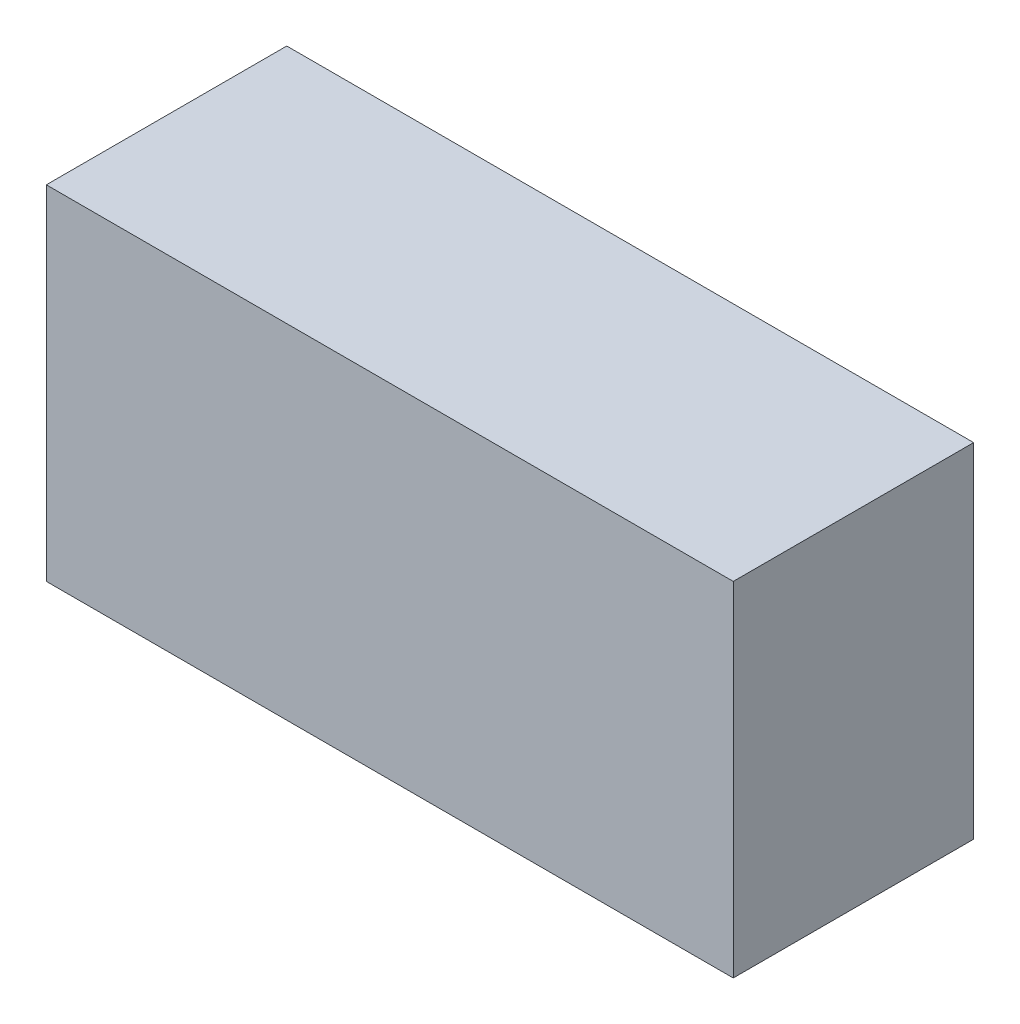
from build123d import *

# Parameters (mm, degrees)
SKETCH_1_W      = 20
SKETCH_1_H      = 10
EXTRUDE_1_DEPTH = 3.5


with BuildPart() as part:
    # 草图1 → 凸台-拉伸1 (new, symmetric)
    with BuildSketch(Plane.XY):
        Rectangle(SKETCH_1_W, SKETCH_1_H)
    extrude(amount=EXTRUDE_1_DEPTH, both=True)


solid = part.part
